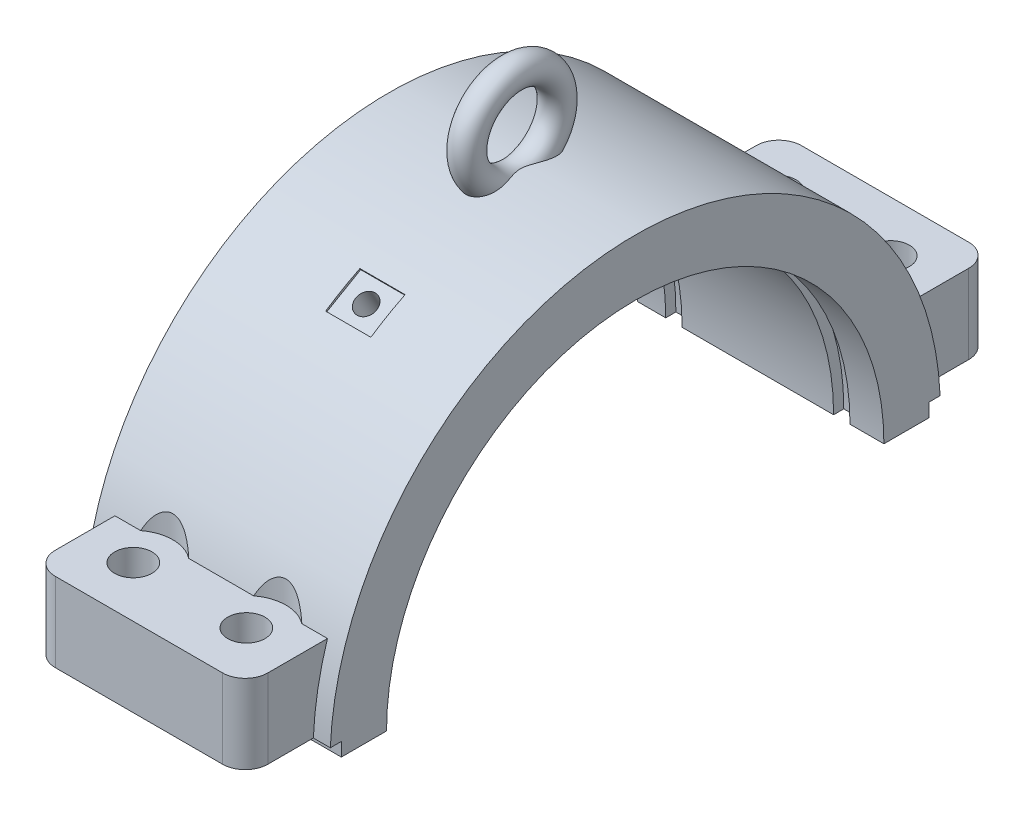
SolidWorks part; units mm, degrees
material "ZG270-500"
ref_plane "Front Plane" through (0, 0, 0) normal (0, 0, 1) x (1, 0, 0)
ref_plane "Top Plane" through (0, 0, 0) normal (0, 1, 0) x (1, 0, 0)
ref_plane "Right Plane" through (0, 0, 0) normal (1, 0, 0) x (0, 0, -1)
sketch "Sketch1" plane through (0, 0, 0) normal (1, 0, 0) x (0, 0, -1)
  line L0 (-323.4956, 0) -> (323.4956, 0) construction
  line L1 (0, 0) -> (0, 289.8169) construction
  line L2 (-270, 0) -> (-220, 0)
  line L3 (220, 0) -> (270, 0)
  arc A0 (220, 0) -> (-220, 0) centre (0, 0) ccw
  arc A1 (270, 0) -> (-270, 0) centre (0, 0) ccw
  point P3 (0, 0)
  dimension "D1" = 440
  dimension "D2" = 540
extrude "Boss-Extrude2" add sketch "Sketch1" along normal mid plane 218
sketch "Sketch4" plane through (0, 0, 0) normal (1, 0, 0) x (0, 0, -1)
  line L0 (-330, 12) -> (-269.7332, 12)
  line L1 (-330, 12) -> (-330, 82)
  line L2 (-330, 82) -> (-257.247, 82)
  line L3 (-270, 0) -> (-220, 0) construction
  line L4 (0, 0) -> (0, 117.0475) construction
  arc A0 (270, 0) -> (-270, 0) centre (0, 0) ccw construction
  arc A1 (-257.247, 82) -> (-269.7332, 12) centre (0, 0) ccw
  dimension "D1" = 12
  dimension "D2" = 70
  dimension "D3" = 330
extrude "Boss-Extrude3" add sketch "Sketch4" along normal mid plane 188
sketch "Sketch5" plane through (0, 82, 0) normal (0, 1, 0) x (1, 0, 0)
  line L0 (0, 0) -> (0, -285) construction
  line L1 (-50, -285) -> (50, -285) construction
  circle A0 centre (50, -285) radius 16.5
  circle A1 centre (-50, -285) radius 16.5
  point P5 (0, -285)
  dimension "D3" = 33
  dimension "D1" = 100
  dimension "D2" = 285
extrude "Cut-Extrude1" cut sketch "Sketch5" against normal through all both and the other way through all
sketch "Sketch6" plane through (0, 0, 0) normal (0, 1, 0) x (1, 0, 0)
  circle A0 centre (-50, -285) radius 35
  circle A1 centre (50, -285) radius 35
  dimension "D1" = 70
extrude "Cut-Extrude2" cut sketch "Sketch6" against normal up to surface (68 mm away) from offset 150
sketch "Sketch7" plane through (0, 0, 0) normal (1, 0, 0) x (0, 0, -1)
  line L0 (-299.2788, 12) -> (-260, 12)
  line L1 (-330, 12) -> (-269.7332, 12) construction
  line L2 (-260, 12) -> (-260, -5.7355)
  line L3 (-260, -5.7355) -> (-299.2788, -5.7355)
  line L4 (-299.2788, -5.7355) -> (-299.2788, 12)
  line L5 (0, 0) -> (0, -107.2673) construction
  dimension "D1" = 260
extrude "Cut-Extrude3" cut sketch "Sketch7" against normal through all both and the other way through all
fillet "Fillet1" radius 20 2 edges at (-94, 47, 330) (94, 47, 330)
mirror "Mirror1" about plane through (0, 0, 0) normal (0, 0, 1) of "Cut-Extrude3", "Boss-Extrude3", "Cut-Extrude1", "Cut-Extrude2", "Fillet1"
sketch "Sketch8" plane through (0, 0, 0) normal (0, 0, 1) x (1, 0, 0)
  line L0 (0, 0) -> (0, 229) construction
  line L1 (-84, 229) -> (-69.5, 229)
  line L2 (-69.5, 229) -> (-69.5, 220)
  line L3 (-69.5, 220) -> (-84, 220)
  line L4 (-84, 220) -> (-84, 229)
  line L6 (109, 0) -> (-109, 0) construction
  line L7 (79, 220) -> (79, 229)
  line L8 (64.5, 220) -> (79, 220)
  line L9 (64.5, 229) -> (64.5, 220)
  line L10 (79, 229) -> (64.5, 229)
  line L11 (0, 0) -> (171.999, 0) construction
  line L12 (109, 12) -> (109, 270) construction
  dimension "D1" = 30
  dimension "D2" = 14.5
  dimension "D3" = 220
  dimension "D4" = 229
  dimension "D5" = 163
  dimension "D6" = 14.5
revolve "Cut-Revolve1" cut sketch "Sketch8" angle 360 about L11
sketch "Sketch9" plane through (0, 0, 0) normal (0, 0, 1) x (1, 0, 0)
  line L0 (0, 0) -> (0, 300) construction
  line L1 (0, 300) -> (128.97, 300) construction
  line L2 (109, 0) -> (-109, 0) construction
  circle A0 centre (0, 340) radius 12.5
  dimension "D2" = 25
  dimension "D3" = 40
  dimension "D1" = 300
revolve "Revolve1" add sketch "Sketch9" angle 360 about L1
sketch "Sketch10" plane through (0, 0, 0) normal (1, 0, 0) x (0, 0, -1)
  line L0 (0, 0) -> (-135, 233.8269) construction
  line L1 (0, 0) -> (0, 321.2312) construction
  line L2 (-149.1554, 223.3448) -> (-118.8446, 240.8448)
  line L3 (-149.1554, 223.3448) -> (-151.1554, 226.8089)
  line L4 (-118.8446, 240.8448) -> (-120.8446, 244.3089)
  line L5 (-151.1554, 226.8089) -> (-120.8446, 244.3089)
  line L6 (-149.1554, 223.3448) -> (-120.8446, 244.3089) construction
  line L7 (-118.8446, 240.8448) -> (-151.1554, 226.8089) construction
  arc A0 (269.7332, 12) -> (-269.7332, 12) centre (0, 0) ccw construction
  dimension "D1" = 30
  dimension "D2" = 2
  dimension "D3" = 35
extrude "Cut-Extrude4" cut sketch "Sketch10" against normal mid plane 40 from offset 5
sketch "Sketch11" plane through (0, 232.0948, 134) normal (0, 0.866, 0.5) x (1, 0, 0)
  line L0 (5, 17.5) -> (5, 0) construction
  line L1 (-15, 17.5) -> (25, 17.5) construction
  line L2 (5, 0) -> (25, 0) construction
  line L3 (25, 17.5) -> (25, -17.5) construction
hole_wizard "M20x1.5 Tapped Hole1" positions "3DSketch1" profile "Sketch12" tap size "M20x1.5" standard "GB" end condition through all
sketch3d "3DSketch1"
  point P0 (5, 232.0948, 134)
cosmetic thread "hole cosmetic thread 1" parameters "D2"=20
sketch "Sketch12" plane through (5, 232.0948, 134) normal (1, 0, 0) x (0, -0.5, 0.866)
  line L0 (0, 0) -> (0, 433)
  line L1 (0, 433) -> (9.25, 433)
  line L2 (9.25, 433) -> (9.25, 0)
  line L5 (9.25, 0) -> (0, 0)
  line L11 (0, -6.35) -> (0, 107.95) construction
  dimension "通孔螺纹孔钻头直径" = 18.5
  dimension "通孔螺纹孔钻头深度" = 433
